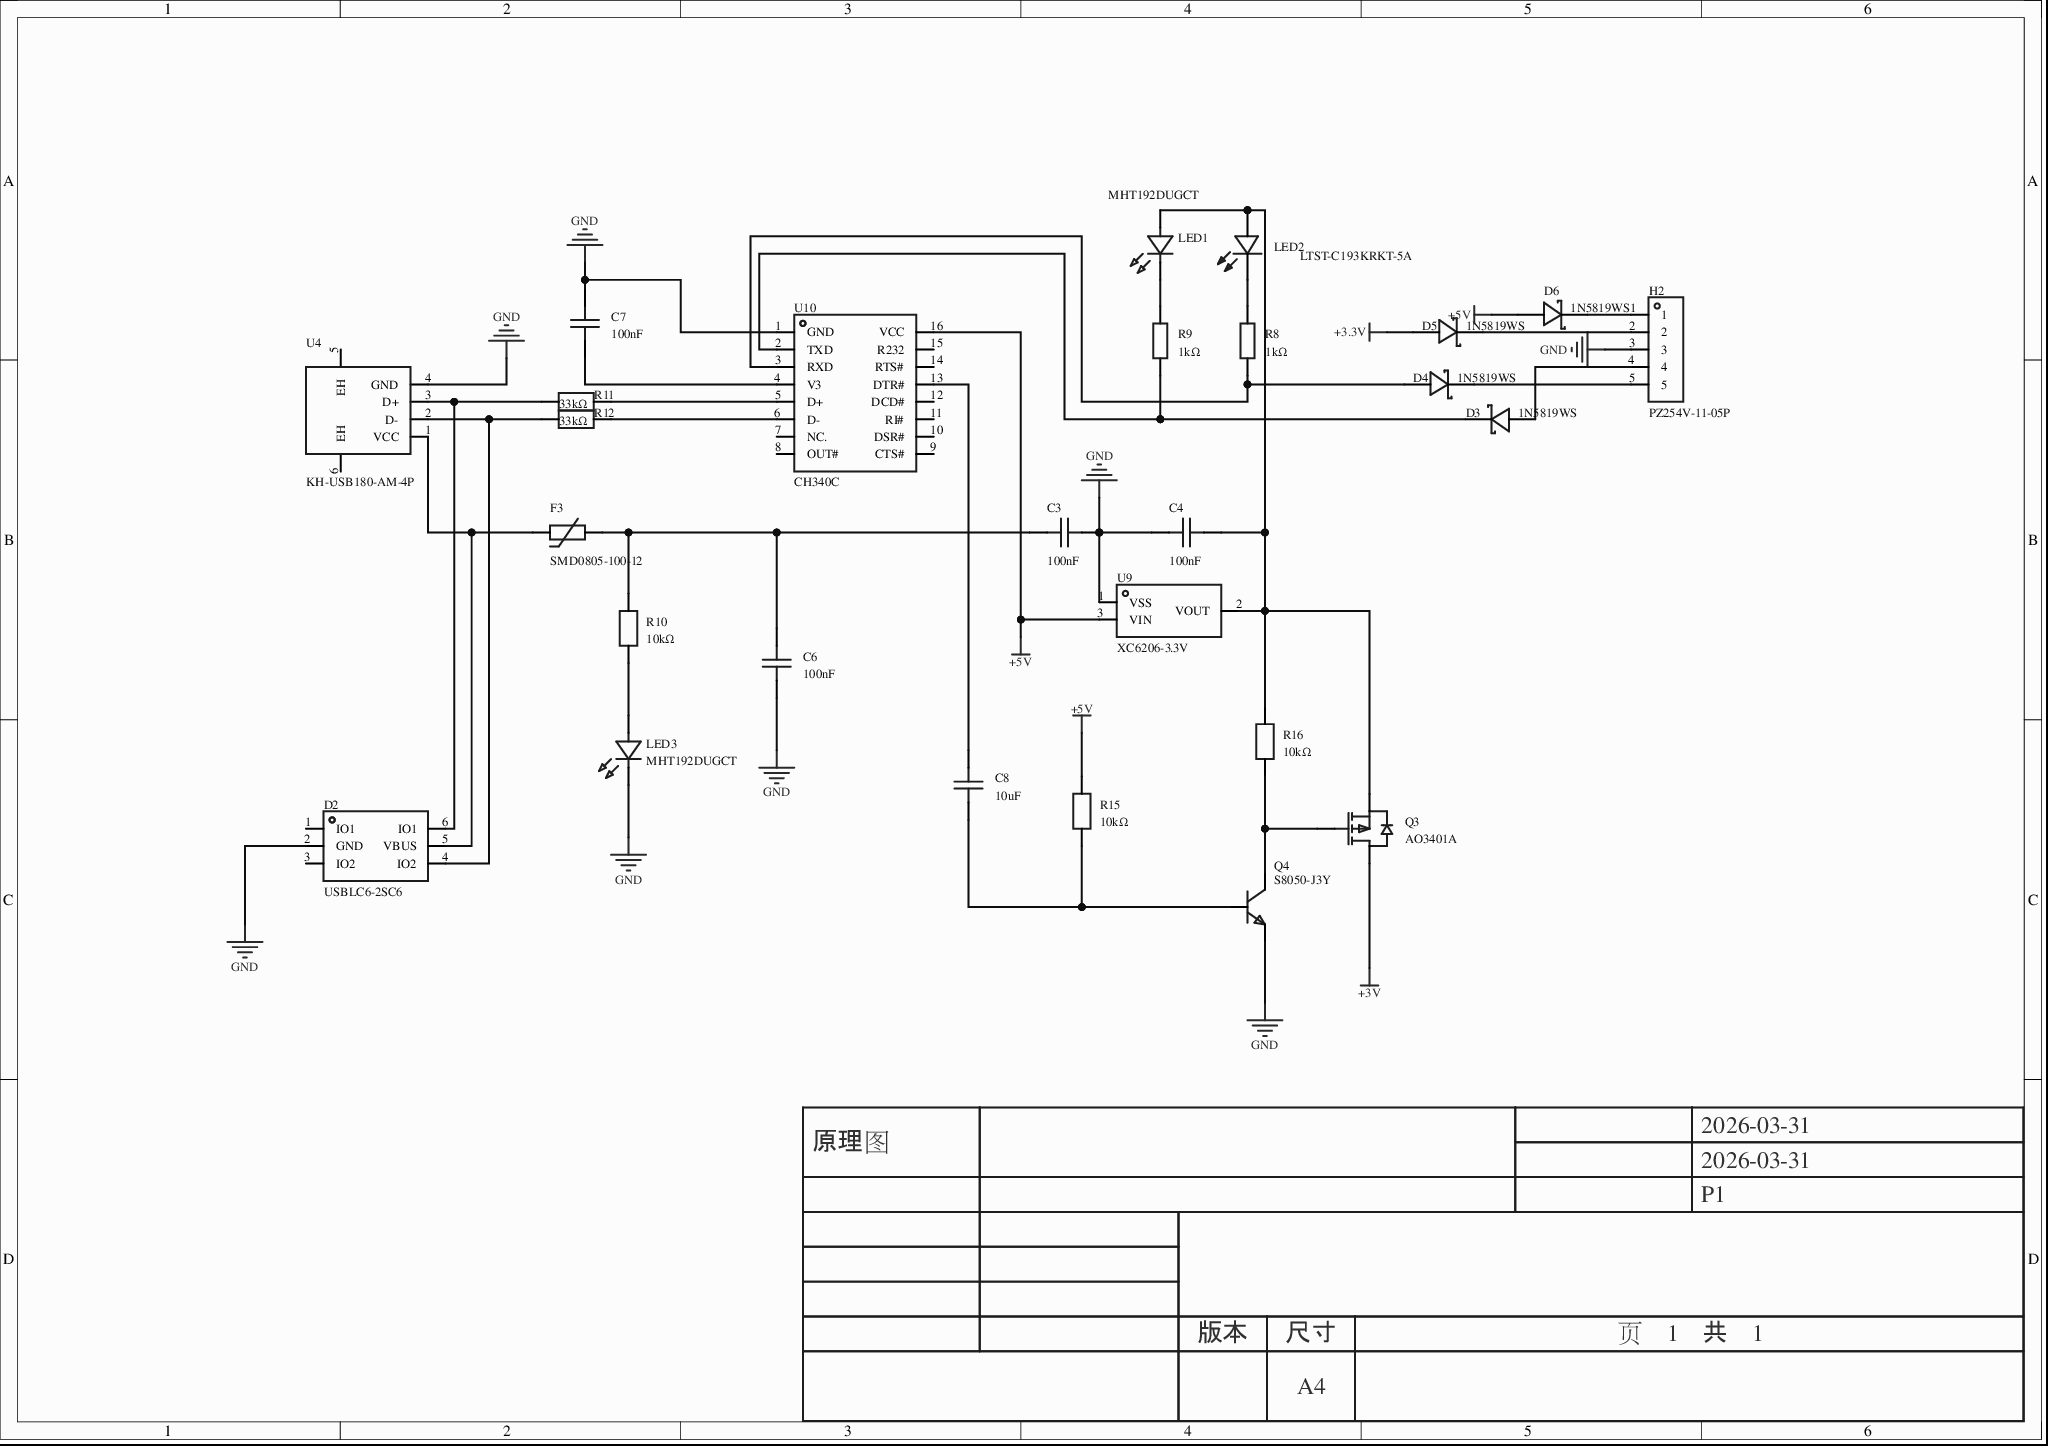
[diagram p0: MISC51088-3.schdoc]
# Altium project MISC51088-2.PrjPcb
1 sheet, 27 parts. Net scope: global (net labels, ports and power ports of the same name join across sheets).
Board file: MISC51088.pcbdoc

## Sheet MISC51088-3.schdoc
size 297 x 209 mm; Version: V1.0; @Project Name: MISC51088; @Update Date: 2026-05-11; @Create Date: 2026-05-11; @Board Name: MISC51088; @Create Time: 08:56:45; @Page Count: 1; @Page No: 1; @Schematic Name: MISC51088; @Update Time: 08:56:45; Size: A4

### Parts
C3  100nF  [C0603]
C4  100nF  [C0603]
C6  100nF  [C0603]
C7  100nF  [C0603]
C8  10uF  [C0603]
D2  USBLC6-2SC6  [SOT-23-6_L2.9-W1.6-P0.95-LS2.8-BL]
D3  1N5819WS  [SOD-323_L1.8-W1.3-LS2.5-RD]
D4  1N5819WS  [SOD-323_L1.8-W1.3-LS2.5-RD]
D5  1N5819WS  [SOD-323_L1.8-W1.3-LS2.5-RD]
D6  1N5819WS  [SOD-323_L1.8-W1.3-LS2.5-RD]
F3  SMD0805-100-12  [R0805]
H2  PZ254V-11-05P  [HDR-TH_5P-P2.54-V-M]
LED1  MHT192DUGCT  [LED0603-RD]
LED2  LTST-C193KRKT-5A  [LED0603-RD]
LED3  MHT192DUGCT  [LED0603-RD]
Q3  AO3401A  [SOT-23_L2.9-W1.3-P1.90-LS2.4-BR]
Q4  S8050-J3Y  [SOT-23-3_L2.9-W1.3-P0.95-LS2.4-BR-1]
R8  1kΩ  [R0603]
R9  1kΩ  [R0603]
R10  10kΩ  [R0603]
R11  33kΩ  [R0603]
R12  33kΩ  [R0603]
R15  10kΩ  [R0603]
R16  10kΩ  [R0603]
U4  KH-USB180-AM-4P  [USB-A-SMD_USB-A-1-TH]
U9  XC6206-3.3V  [SSOT-3_L2.9-W1.6-P0.95-LS2.8-BR]
U10  CH340C  [SOP-16_L10.0-W3.9-P1.27-LS6.0-BL]

### Nets
+3.3V: D5.2(A)
+3V: Q3.3(D)
+5V: D6.2(A) R15.2 U9.3(VIN) U10.16(VCC)
GND: C3.2 C4.1 C6.1 C7.2 D2.2(GND) H2.3 LED3.1(K) Q4.2(E) U4.4(GND) U9.1(VSS) U10.1(GND)
NetC3_1: C3.1 C6.2 F3.2 R10.2
NetC4_2: C4.2 LED1.2(A) LED2.2(A) Q3.2(S) R16.2 U9.2(VOUT)
NetC7_1: C7.1 U10.4(V3)
NetC8_1: C8.1 Q4.1(B) R15.1
NetC8_2: C8.2 U10.13(DTR#)
NetD2_4: D2.4(IO2) R12.1 U4.2(D-)
NetD2_5: D2.5(VBUS) F3.1 U4.1(VCC)
NetD2_6: D2.6(IO1) R11.1 U4.3(D+)
NetD3_1: D3.1(K) R9.1 U10.2(TXD)
NetD3_2: D3.2(A) H2.4
NetD4_1: D4.1(K) H2.5
NetD4_2: D4.2(A) R8.1 U10.3(RXD)
NetD5_1: D5.1(K) H2.2
NetD6_1: D6.1(K) H2.1
NetLED1_1: LED1.1(K) R9.2
NetLED2_1: LED2.1(K) R8.2
NetLED3_2: LED3.2(A) R10.1
NetQ3_1: Q3.1(G) Q4.3(C) R16.1
NetR11_2: R11.2 U10.5(D+)
NetR12_2: R12.2 U10.6(D-)

Not connected (* = marked no-connect by the designer): D2 1(IO1) 3(IO2); U4 5(EH) 6(EH); U10 7(NC.) 8(OUT#) 9(CTS#) 10(DSR#) 11(RI#) 12(DCD#) 14(RTS#) 15(R232)

### Notes on the sheet
- 2026-03-31
- 原理图
- P1
- 版本
- 尺寸
- A4
- 页    1    共    1

### Library data of the parts
C3 C4 C6 = CGA0603X7R104K500JT: 容值:100nF;精度:±10%;额定电压:50V;温度系数:X7R;; Manufacturer: HRE(芯声); AddInBom: yes; Tolerance: ±10%; Voltage Rating: 50V; Temperature Coefficient: X7R; ModelId: ac125912035d415993ca9572d50418b10819f05c4eef4c71ace90d822a990e87; ModelName: C0603_L1.6-W0.8-H0.8; ModelTransform: 62.992,31.496,0,0,0,0,0,0,0; Device: CGA0603X7R104K500JT; Symbol: CGA0603X7R104K500JT; FootprintName: C0603; LCSC Part Name: 100nF ±10% 50V; SupplierPart: C6119867; ManufacturerPart: CGA0603X7R104K500JT; Supplier Footprint: 0603; JLCPCB Part Class: Extended Part; Datasheet: https://item.szlcsc.com/datasheet/CGA0603X7R104K500JT/7062573.html; Supplier: LCSC; ConvertToPcb: yes; Value: 100nF
C7 = CC0603KRX7R9BB104: 容值:100nF;精度:±10%;额定电压:50V;温度系数:X7R;; Manufacturer: YAGEO(国巨); AddInBom: yes; Tolerance: ±10%; Voltage Rating: 50V; Temperature Coefficient: X7R; ModelId: ac125912035d415993ca9572d50418b10819f05c4eef4c71ace90d822a990e87; ModelName: C0603_L1.6-W0.8-H0.8; ModelTransform: 62.992,31.496,0,0,0,0,0,0,0; Device: CC0603KRX7R9BB104; Symbol: CC0603KRX7R9BB104; FootprintName: C0603; LCSC Part Name: 100nF ±10% 50V; SupplierPart: C14663; ManufacturerPart: CC0603KRX7R9BB104; Supplier Footprint: 0603; JLCPCB Part Class: Basic Part; Datasheet: https://item.szlcsc.com/datasheet/CC0603KRX7R9BB104/15331.html; Supplier: LCSC; ConvertToPcb: yes; Value: 100nF
C8 = CL10A106MA8NRNC: 容值:10uF;精度:±20%;额定电压:25V;温度系数:X5R;; Manufacturer: SAMSUNG(三星); AddInBom: yes; Tolerance: ±20%; Voltage Rating: 25V; Temperature Coefficient: X5R; ModelId: ac125912035d415993ca9572d50418b10819f05c4eef4c71ace90d822a990e87; ModelName: C0603_L1.6-W0.8-H0.8; ModelTransform: 62.992,31.496,0,0,0,0,0,0,0; Device: CL10A106MA8NRNC; Symbol: CL10A106MA8NRNC; FootprintName: C0603; LCSC Part Name: 10uF ±20% 25V; SupplierPart: C96446; ManufacturerPart: CL10A106MA8NRNC; Supplier Footprint: 0603; JLCPCB Part Class: Basic Part; Datasheet: https://item.szlcsc.com/datasheet/CL10A106MA8NRNC/97651.html; Supplier: LCSC; ConvertToPcb: yes; Value: 10uF
D2 = USBLC6-2SC6_C2827654: 极性:单向;反向截止电压(Vrwm):5V;钳位电压:12V;峰值脉冲电流(Ipp):6A;峰值脉冲功率(Ppp):150W;击穿电压:6V;; Manufacturer: TECH PUBLIC(台舟); AddInBom: yes; Polarity: 单向; Reverse Stand-Off Voltage (Vrwm): 5V; Clamping Voltage: 12V; Peak Pulse Current (Ipp): 6A; Peak Pulse Power Dissipation (Ppp): 150W; Voltage - Breakdown: 6V; Reverse Leakage Current (Ir): 80nA; Number of Channels: 双路; level of protection: IEC 61000-4-2；IEC 61000-4-4；IEC 61000-4-5; Type: ESD; Junction Capacitance: 0.35pF; ModelId: 18da8f6c14a34920b3e136b5c401a1190819f05c4eef4c71ace90d822a990e87; ModelName: SOT-23-6_L2.9-W1.6-H1.5-LS2.8-P0.95; ModelTransform: 110.236,113.364,0,90,0,0,0.0005,0.0005,0; Device: USBLC6-2SC6_C2827654; Symbol: USBLC6-2SC6_C2827654; FootprintName: SOT-23-6_L2.9-W1.6-P0.95-LS2.8-BL; LCSC Part Name: ESD，可防30kV静电; SupplierPart: C2827654; ManufacturerPart: USBLC6-2SC6; Supplier Footprint: SOT-23-6; JLCPCB Part Class: Extended Part; Datasheet: https://item.szlcsc.com/datasheet/USBLC6-2SC6/2973336.html; Supplier: LCSC; ConvertToPcb: yes; Operating Temperature: -55℃~+125℃
D3-D6 = 1N5819WS_C191023: 正向压降(Vf):600mV@1A;直流反向耐压(Vr):40V;整流电流:1A;; Manufacturer: Hottech(合科泰); AddInBom: yes; Voltage - DC Reverse(Vr): 40V; Current - Rectified: 1A; Non-Repetitive Peak Forward Surge Current: 25A; ModelId: 7459fe65e23146c0a8d836e46a0add720819f05c4eef4c71ace90d822a990e87; ModelTransform: 104.3305,51.181,0,0,0,0,0,0,0; Device: 1N5819WS_C191023; Symbol: 1N5819WS; FootprintName: SOD-323_L1.8-W1.3-LS2.5-RD; LCSC Part Name: 电压:40V 电流:1A; SupplierPart: C191023; ManufacturerPart: 1N5819WS; Supplier Footprint: SOD-323; JLCPCB Part Class: Basic Part; Datasheet: https://item.szlcsc.com/datasheet/1N5819WS/213850.html; Supplier: LCSC; ConvertToPcb: yes; Voltage - Forward(Vf@If): 600mV@1A; ModelName: SOD-323_L1.8-W1.3-LS2.5-RD
F3 = SMD0805-100-12: 耐压(Vmax):12V;最大电流(Imax):40A;保持电流(Ihold):1A;跳闸电流(Itrip):2A;; Manufacturer: R+O(宏嘉诚); AddInBom: yes; Voltage - Max: 12V; Current - Max: 40A; Hold Current: 1A; Trip Current: 2A; Power Dissipation: 600mW; Resistance - Initial (Ri) (Min): 40mΩ; Resistance - Post Trip (R1) (Max): 270mΩ; Time to Trip(Max): 300ms; ModelId: 37a81e68749a4138bd2dfa6897b24b850819f05c4eef4c71ace90d822a990e87; ModelName: R0805_L2.0-W1.3-H0.6; ModelTransform: 78.74,51.181,0,0,0,0,0,-0.0005,0; Device: SMD0805-100-12; Symbol: SMD0805-100-12; FootprintName: R0805; LCSC Part Name: 12V 1A; SupplierPart: C46640991; ManufacturerPart: SMD0805-100-12; Supplier Footprint: 0805; JLCPCB Part Class: Extended Part; Datasheet: https://item.szlcsc.com/datasheet/SMD0805-100-12/48798697.html; Supplier: LCSC; ConvertToPcb: yes; Operating Temperature: -40℃~+85℃; Length: 2.2mm; Width: 1.5mm
H2 = PZ254V-11-05P: 插针结构:1x5P;间距:2.54mm;行距:-;圆针/方针:方针;安装方式:直插;排数:单排;总PIN位数:5P;额定电流:3A;额定电压:250V;配合针长度:6mm;塑高:2.5mm;端接针长度:3mm;触头材质:黄铜;触头镀层:-;工作温度:-40℃~+105℃;颜色:黑色;; Manufacturer: XFCN(兴飞); AddInBom: yes; Pin Structure: 1x5P; Pitch: 2.54mm; Circluar Pins/Square Pins: 方针; Current Rating: 3A; Voltage Rating (Max): 250V; ModelId: 47d466e4a34f4fc5bc626cf773a24dd50819f05c4eef4c71ace90d822a990e87; ModelName: HDR-TH_5P-P2.54-M-LI-1X5P; ModelTransform: 499.999,100,0,0,0,0,0,0,-118.11; Device: PZ254V-11-05P; Symbol: PZ254V-11-05P; FootprintName: HDR-TH_5P-P2.54-V-M; LCSC Part Name: 1x5P 间距:2.54mm 方针 直插; SupplierPart: C492404; ManufacturerPart: PZ254V-11-05P; Supplier Footprint: 插件,P=2.54mm; JLCPCB Part Class: Extended Part; Datasheet: https://item.szlcsc.com/datasheet/PZ254V-11-05P/502960.html; Supplier: LCSC; ConvertToPcb: yes; Row Spacing: -; Mounting Type: 直插; Number of Rows: 单排; Number of Pins: 5P; Length of Mating Pin: 6mm; Insulation Height: 2.5mm; Length of End Connection Pin: 3mm; Contact Material: 黄铜; Contact Plating: -; Operating Temperature: -40℃~+105℃; Color: 黑色
LED1 LED3 = MHT192DUGCT: 灯头类型:-;发光颜色:翠绿色;正向压降(Vf):2.3V~2.8V;功率:60mW;正向电流:5mA;波长:515nm~530nm;二极管配置:独立二极管;透镜颜色:无色透明透镜;色温:-;发光强度:565mcd;发光角度:120°;载带方式:-;工作温度:-40℃~+85℃;; Manufacturer: MEIHUA(美华); AddInBom: yes; Illumination Color: 翠绿色; Power(Watts): 60mW; Forward Current: 5mA; Peak Wavelength: 518nm; Diode Configuration: 独立二极管; Lens Color: 无色透明透镜; Luminous Intensity: 565mcd; Viewing Angle: 120°; ModelId: 1f0d29a91be547639d425604e9b96ebb0819f05c4eef4c71ace90d822a990e87; ModelTransform: 63.7794,32.283,0,0,0,0,0,0,0; Device: MHT192DUGCT; Symbol: MHT192DUGCT; FootprintName: LED0603-RD; LCSC Part Name: 0603正贴翠绿色光0.6T; SupplierPart: C7470862; ManufacturerPart: MHT192DUGCT; Supplier Footprint: 0603; JLCPCB Part Class: Extended Part; Datasheet: https://item.szlcsc.com/datasheet/MHT192DUGCT/8521967.html; Supplier: LCSC; ConvertToPcb: yes; Lamp Holder Type: -; Voltage - Forward(Vf): 2.3V~2.8V; Wavelength - Dominant: 515nm~530nm; Color Temperature: -; Mounting Style: -; Operating Temperature: -40℃~+85℃; ModelName: LED0603-RD
LED2 = LTST-C193KRKT-5A: 灯头类型:-;发光颜色:红色;正向压降(Vf):2V;功率:50mW;正向电流:20mA;波长:631nm;二极管配置:独立二极管;透镜颜色:无色透明透镜;色温:-;发光强度:26.05mcd;发光角度:130°;载带方式:-;工作温度:-30℃~+85℃;; Manufacturer: LITEON(光宝); AddInBom: yes; Illumination Color: 红色; Voltage - Forward(Vf): 2V; Power(Watts): 50mW; Forward Current: 20mA; Wavelength - Dominant: 631nm; Peak Wavelength: 639nm; Diode Configuration: 独立二极管; Lens Color: 无色透明透镜; Viewing Angle: 130°; ModelId: 1f0d29a91be547639d425604e9b96ebb0819f05c4eef4c71ace90d822a990e87; ModelTransform: 63.7794,32.283,0,0,0,0,0,0,0; Device: LTST-C193KRKT-5A; Symbol: LTST-C193KRKT-5A; FootprintName: LED0603-RD; LCSC Part Name: 红灯; SupplierPart: C157741; ManufacturerPart: LTST-C193KRKT-5A; Supplier Footprint: 0603; JLCPCB Part Class: Extended Part; Datasheet: https://item.szlcsc.com/datasheet/LTST-C193KRKT-5A/169089.html; Supplier: LCSC; ConvertToPcb: yes; Lamp Holder Type: -; Color Temperature: -; Luminous Intensity: 26.05mcd; Mounting Style: -; Operating Temperature: -30℃~+85℃; ModelName: LED0603-RD
Q3 = AO3401A_C15127: 数量:1个P沟道;漏源电压(Vdss):30V;连续漏极电流(Id):4A;导通电阻(RDS(on)):47mΩ@10V；85mΩ@2.5V；60mΩ@4.5V;耗散功率(Pd):-;阈值电压(Vgs(th)):900mV@250uA;; Manufacturer: AOS; AddInBom: yes; Number: 1个P沟道; Drain to Source Voltage: 30V; Current - Continuous Drain(Id): 4A; Gate Charge(Qg): 14nC@10V; Input Capacitance(Ciss): 645pF; Reverse Transfer Capacitance (Crss@Vds): 55pF; Output Capacitance(Coss): 80pF; ModelId: c62791f0466c4ae2a892c056b845b0ca0819f05c4eef4c71ace90d822a990e87; ModelName: SOT-23-3P_L2.9-W1.3-H1.0-LS2.4-P0.95; ModelTransform: 98.425,114.173,0,180,0,0,0.0005,-0.0005,0; Device: AO3401A_C15127; Symbol: AO3401A; FootprintName: SOT-23_L2.9-W1.3-P1.90-LS2.4-BR; LCSC Part Name: 1个P沟道 耐压:30V 电流:4A; SupplierPart: C15127; ManufacturerPart: AO3401A; Supplier Footprint: SOT-23; JLCPCB Part Class: Basic Part; Datasheet: https://item.szlcsc.com/datasheet/AO3401A/15801.html; Supplier: LCSC; ConvertToPcb: yes; RDS(on): 47mΩ@10V；85mΩ@2.5V；60mΩ@4.5V; Pd - Power Dissipation: -; Gate Threshold Voltage (Vgs(th)): 900mV@250uA; Operating Temperature: -; Type: -
Q4 = S8050-J3Y: 晶体管类型:NPN;集电极电流(Ic):300mA;集射极击穿电压(Vceo):25V;耗散功率(Pd):300mW;直流电流增益(hFE):350@50mA,1V;; Manufacturer: JSMSEMI(杰盛微); Symbol: S8050-J3Y_C18221467; AddInBom: yes; type: NPN; Current - Collector(Ic): 300mA; Collector - Emitter Voltage VCEO: 25V; Pd - Power Dissipation: 300mW; Transition frequency(fT): 150MHz; Current - Collector Cutoff: 100nA; Vce Saturation(VCE(sat)): 600mV@500mA,50mA; Emitter-Base Voltage(Vebo): 5V; ModelId: ef41b3e5dd9e422d964387bb3b69faa10819f05c4eef4c71ace90d822a990e87; ModelTransform: 94.488,114.173,0,0,0,0,0,0,0; Device: S8050-J3Y; FootprintName: SOT-23-3_L2.9-W1.3-P0.95-LS2.4-BR-1; LCSC Part Name: hFE:200-300 NPN 电流:300mA 电压:25V; SupplierPart: C18221467; ManufacturerPart: S8050-J3Y; Supplier Footprint: SOT-23; JLCPCB Part Class: Extended Part; Datasheet: https://item.szlcsc.com/datasheet/S8050-J3Y/19402088.html; Supplier: LCSC; ConvertToPcb: yes; DC Current Gain: 350@50mA,1V; Operating Temperature: -; ModelName: SOT-23-3_L2.9-W1.3-P0.95-LS2.4-BR-1
R8 R9 = 0603WAF1001T5E: 电阻类型:厚膜电阻;阻值:1kΩ;精度:±1%;功率:100mW;工作电压:75V;温度系数:±100ppm/℃;; Manufacturer: UNI-ROYAL(厚声); AddInBom: yes; Tolerance: ±1%; Power(Watts): 100mW; Voltage-Supply(Max): 75V; ModelId: fc143cca1e79419f9cd78b61e9279f080819f05c4eef4c71ace90d822a990e87; ModelTransform: 31.8897,63.7794,0,90,0,0,0,0,0; Device: 0603WAF1001T5E; Symbol: 0603WAF1001T5E; FootprintName: R0603; LCSC Part Name: 1kΩ ±1% 100mW 厚膜电阻; SupplierPart: C21190; ManufacturerPart: 0603WAF1001T5E; Supplier Footprint: 0603; JLCPCB Part Class: Basic Part; Datasheet: https://item.szlcsc.com/datasheet/0603WAF1001T5E/21904.html; Supplier: LCSC; ConvertToPcb: yes; Type: 厚膜电阻; Value: 1kΩ; Temperature Coefficient: ±100ppm/℃; Operating Temperature: -55℃~+155℃; ModelName: R0603
R10 R15 R16 = FRC0603F1002TS: 电阻类型:厚膜电阻;阻值:10kΩ;精度:±1%;功率:100mW;工作电压:75V;温度系数:±100ppm/℃;; Manufacturer: FOJAN(富捷); AddInBom: yes; Tolerance: ±1%; Power(Watts): 100mW; Voltage-Supply(Max): 75V; ModelId: fc143cca1e79419f9cd78b61e9279f080819f05c4eef4c71ace90d822a990e87; ModelTransform: 31.8897,63.7794,0,90,0,0,0,0,0; Device: FRC0603F1002TS; Symbol: FRC0603F1002TS; FootprintName: R0603; LCSC Part Name: 10kΩ ±1% 100mW 厚膜电阻; SupplierPart: C2906982; ManufacturerPart: FRC0603F1002TS; Supplier Footprint: 0603; JLCPCB Part Class: Extended Part; Supplier: LCSC; ConvertToPcb: yes; Type: 厚膜电阻; Value: 10kΩ; Temperature Coefficient: ±100ppm/℃; Operating Temperature: -55℃~+155℃; ModelName: R0603
R11 R12 = FRC0603F3302TS: 电阻类型:厚膜电阻;阻值:33kΩ;精度:±1%;功率:100mW;工作电压:75V;温度系数:±100ppm/℃;; Manufacturer: FOJAN(富捷); AddInBom: yes; Tolerance: ±1%; Power(Watts): 100mW; Voltage-Supply(Max): 75V; ModelId: fc143cca1e79419f9cd78b61e9279f080819f05c4eef4c71ace90d822a990e87; ModelTransform: 31.8897,63.7794,0,90,0,0,0,0,0; Device: FRC0603F3302TS; Symbol: FRC0603F3302TS; FootprintName: R0603; LCSC Part Name: 33kΩ ±1% 100mW 厚膜电阻; SupplierPart: C2907028; ManufacturerPart: FRC0603F3302TS; Supplier Footprint: 0603; JLCPCB Part Class: Extended Part; Supplier: LCSC; ConvertToPcb: yes; Type: 厚膜电阻; Value: 33kΩ; Temperature Coefficient: ±100ppm/℃; Operating Temperature: -55℃~+155℃; ModelName: R0603
U4 = KH-USB180-AM-4P: 连接器类型:Type-A;协议标准:USB 2.0;公母:公;安装方式:卧贴;触点数量:4P;端口数量:1;额定电流 - 电源:-;工作温度:-;; Manufacturer: kinghelm(金航标); AddInBom: yes; Connector Type: Type-A; Protocol Standard: USB 2.0; Gender: 公; Number of Contacts: 4P; Number of Ports: 1; ModelId: f6f4a0fb4b8446c28a8faf79888527ee0819f05c4eef4c71ace90d822a990e87; ModelName: USB-A-SMD_4P-L12.0-W18.8-H4.5-LS12.8; ModelTransform: 499.10806,816.927,0,90,0,0,341.534,0,-98.425; Device: KH-USB180-AM-4P; Symbol: KH-USB180-AM-4P; FootprintName: USB-A-SMD_USB-A-1-TH; LCSC Part Name: Type-A 公 卧贴; SupplierPart: C2828094; ManufacturerPart: KH-USB180-AM-4P; Supplier Footprint: SMD; JLCPCB Part Class: Extended Part; Datasheet: https://item.szlcsc.com/datasheet/KH-USB180-AM-4P/2975546.html; Supplier: LCSC; ConvertToPcb: yes; Mounting Type: 卧贴; Current Rating-Power: -; Length: 18.8mm; Operating Temperature: -
U9 = XC6206-3.3V: 输出类型:固定;工作电压:6V;输出电压:3.3V;输出电流:250mA;电源纹波抑制比(PSRR):-;输出极性:正极;; Manufacturer: YONGYUTAI(永裕泰); Add into BOM: yes; 3D Model: e421836395974fbe850bab305eea4e31; 3D Model Transform: 114.96,98.8187,0,90,0,0,0,0,0; Output Type: 固定; Voltage - Supply: 6V; Output Voltage: 3.3V; Output Current: 250mA; Voltage Dropout: 400mV@(200mA); standby current: 3uA; Output Configuration: 正极; Number of Outputs: 1; Device: XC6206-3.3V; Symbol: XC6206-3.3V; Convert to PCB: yes; LCSC Part Name: 3.3V 250mA 6V; Supplier Part: C2891841; Manufacturer Part: XC6206-3.3V; Supplier Footprint: SOT-23-3L; JLCPCB Part Class: Extended Part; Datasheet: https://item.szlcsc.com/datasheet/XC6206-3.3V/3119760.html; Supplier: LCSC; Power Supply Rejection Ratio (PSRR): -; Noise: -; Features: 过流保护; Operating Temperature: -40℃~+125℃@(Tj); FootprintName: SSOT-3_L2.9-W1.6-P0.95-LS2.8-BR; ModelName: SSOT-3_L2.9-W1.6-P0.95-LS2.8-BR
U10 = CH340C: 应用功能:收发器;USB协议版本:USB 2.0;数据速率:2Mbps;; Manufacturer: WCH(南京沁恒); AddInBom: yes; Applications Function: 收发器; USB Protocol: USB 2.0; Voltage - Supply: 3.3V；5V; Data Rate: 2Mbps; Current - Supply: 7mA; Supply Current (Iq): 50uA; ModelId: 3361a6792abf4a8f8fbca4f1924a67ee0819f05c4eef4c71ace90d822a990e87; ModelName: SOP-16_L9.9-W3.9-H1.5-LS6.0-P1.27; ModelTransform: 240.39054,393.7,0,90,0,0,0,0,0; Device: CH340C; Symbol: CH340C; FootprintName: SOP-16_L10.0-W3.9-P1.27-LS6.0-BL; LCSC Part Name: USB转串口芯片; SupplierPart: C84681; ManufacturerPart: CH340C; Supplier Footprint: SOP-16; JLCPCB Part Class: Extended Part; Datasheet: https://item.szlcsc.com/datasheet/CH340C/85852.html; Supplier: LCSC; ConvertToPcb: yes; Operating Temperature: -20℃~+70℃